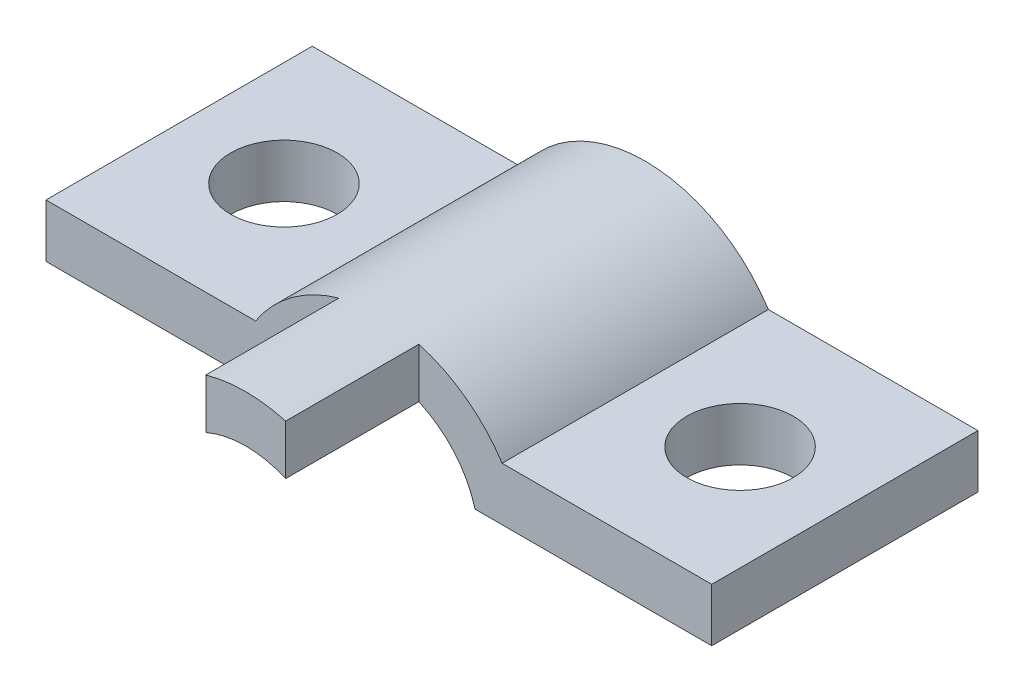
from build123d import *

# Parameters (mm, degrees)
EXTRUDE_5_DEPTH     = 30
SKETCH_5_W          = 22
SKETCH_5_H          = 10
CUT_EXTRUDE_7_DEPTH = 41.081973509
SKETCH_6_R          = 4
CUT_EXTRUDE_8_DEPTH = 40.374028275


with BuildPart() as part:
    # 草图1 → 拉伸5 (new body)
    with BuildSketch(Plane.XY):
        with BuildLine():
            Line((7.228416147, 4), (25, 4))
            Line((25, 4), (25, 8))
            Line((25, 8), (9.256881183, 8))
            ThreePointArc((9.256881183, 8), (0, 13.031312217), (-9.256881183, 8))
            Line((-9.256881183, 8), (-25, 8))
            Line((-25, 8), (-25, 4))
            Line((-25, 4), (-7.228416147, 4))
            ThreePointArc((-7.228416147, 4), (0, 9.5), (7.228416147, 4))
        make_face()
    extrude(amount=EXTRUDE_5_DEPTH)

    # 草图5 → 拉伸7 (cut, through all)
    with BuildSketch(Plane.XZ.offset(-4)):
        with Locations((-14, 25)):
            Rectangle(SKETCH_5_W, SKETCH_5_H)
        with Locations((14, 25)):
            Rectangle(SKETCH_5_W, SKETCH_5_H)
    extrude(amount=-CUT_EXTRUDE_7_DEPTH, mode=Mode.SUBTRACT)

    # 草图6 → 拉伸8 (cut, through all)
    with BuildSketch(Plane(origin=(0, 8, 0), x_dir=(1, 0, 0), z_dir=(0, 1, 0))):
        with Locations(Location((-17.128440592, -10, 0), (0, 0, 180))):
            Circle(SKETCH_6_R)
        with Locations(Location((17.128440592, -10, 0), (0, 0, 180))):
            Circle(SKETCH_6_R)
    extrude(amount=-CUT_EXTRUDE_8_DEPTH, mode=Mode.SUBTRACT)


solid = part.part
